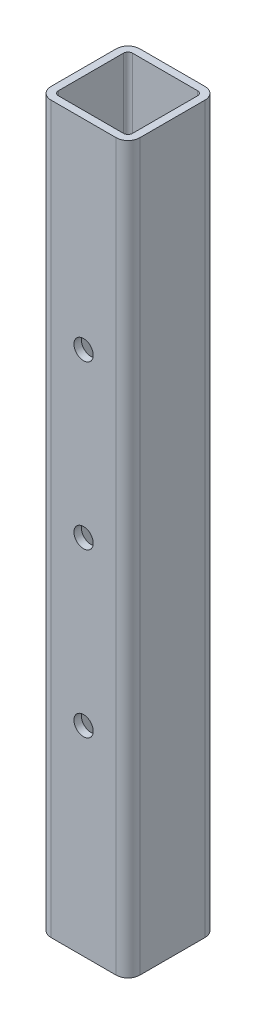
from build123d import *

# Parameters (mm, degrees)
GB_T6728_2002_120_120_10_1_DEPTH = 980
HOLE_WIZARD_26_1_D               = 26


with BuildPart() as part:
    # Sketch12 → 结构用冷弯空心方钢(gb t6728-2002) 120×120×10(1) (new body)
    with BuildSketch(Plane(origin=(0, 0, 0), x_dir=(-1, 0, 0), z_dir=(0, 1, 0))):
        with BuildLine():
            Line((-44, -60), (44, -60))
            ThreePointArc((44, -60), (55.313708499, -55.313708499), (60, -44))
            Line((60, -44), (60, 44))
            ThreePointArc((60, 44), (55.313708499, 55.313708499), (44, 60))
            Line((44, 60), (-44, 60))
            ThreePointArc((-44, 60), (-55.313708499, 55.313708499), (-60, 44))
            Line((-60, 44), (-60, -44))
            ThreePointArc((-60, -44), (-55.313708499, -55.313708499), (-44, -60))
        make_face()
        with BuildLine():
            Line((-44, -50), (44, -50))
            ThreePointArc((44, -50), (48.242640687, -48.242640687), (50, -44))
            Line((50, -44), (50, 44))
            ThreePointArc((50, 44), (48.242640687, 48.242640687), (44, 50))
            Line((44, 50), (-44, 50))
            ThreePointArc((-44, 50), (-48.242640687, 48.242640687), (-50, 44))
            Line((-50, 44), (-50, -44))
            ThreePointArc((-50, -44), (-48.242640687, -48.242640687), (-44, -50))
        make_face(mode=Mode.SUBTRACT)
    extrude(amount=GB_T6728_2002_120_120_10_1_DEPTH)

    # Ø26 直径孔1 (through all)
    with Locations(Plane.XY.offset(60)):
        with Locations((0, 710), (0, 490), (0, 270)):
            Hole(HOLE_WIZARD_26_1_D / 2)


solid = part.part
